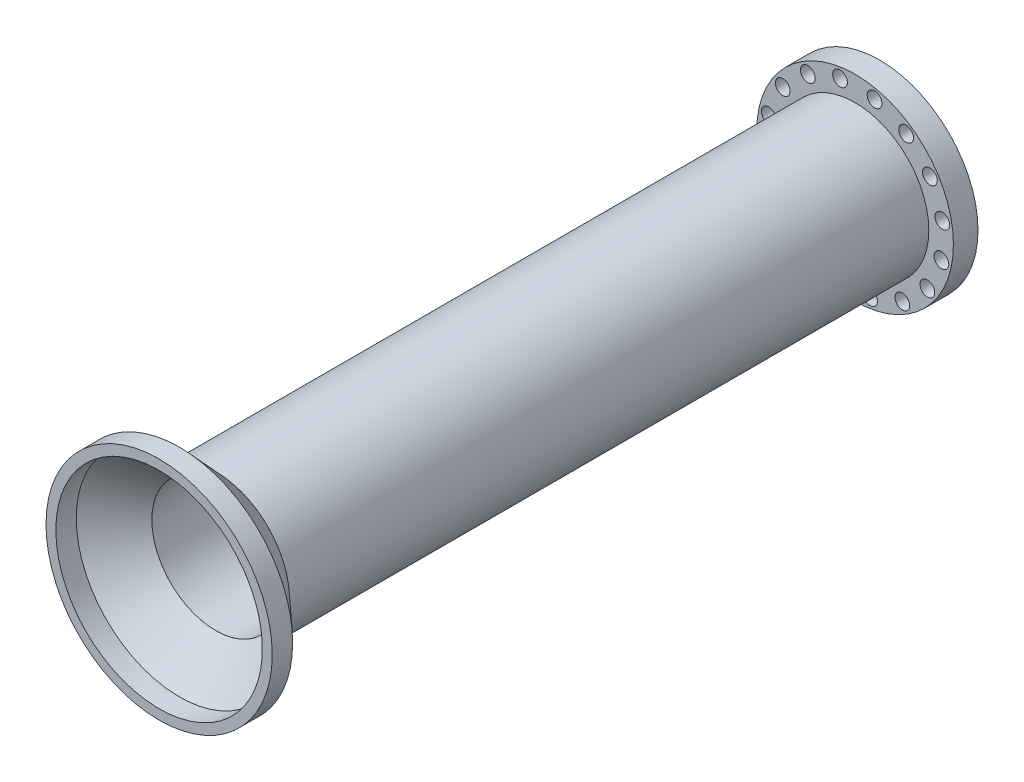
SolidWorks part; units mm, degrees
ref_plane "Front Plane" through (0, 0, 0) normal (0, 0, 1) x (1, 0, 0)
ref_plane "Top Plane" through (0, 0, 0) normal (0, 1, 0) x (1, 0, 0)
ref_plane "Right Plane" through (0, 0, 0) normal (1, 0, 0) x (0, 0, -1)
sketch "Sketch1" plane through (0, 0, 0) normal (0, 0, 1) x (1, 0, 0)
  line L1 (5, 78.5631) -> (35, 78.5631) construction
  circle A0 centre (20, 55.8305) radius 20
  circle A1 centre (20, 55.8305) radius 15
  point P5 (20, 78.5631)
  dimension "D1" = 40
  dimension "D2" = 30
extrude "Boss-Extrude1" add sketch "Sketch1" along normal blind 5 contours A1 | A0 A1
sketch "Sketch2" plane through (0, 0, 5) normal (0, 0, 1) x (1, 0, 0)
  circle A0 centre (20, 55.8305) radius 15
  circle A1 centre (20, 55.8305) radius 20 construction
  dimension "D1" = 5
extrude "Boss-Extrude2" add sketch "Sketch2" along normal blind 130
sketch "Sketch3" plane through (0, 0, 135) normal (0, 0, 1) x (1, 0, 0)
  circle A0 centre (20, 55.8305) radius 13
  circle A1 centre (20, 55.8305) radius 15 construction
  dimension "D1" = 2
extrude "Cut-Extrude1" cut sketch "Sketch3" against normal up to surface (130 mm away) and the other way through all up to face at (35, 55.8305, 5)
sketch "Sketch4" plane through (0, 0, 5) normal (0, 0, 1) x (1, 0, 0)
  circle A0 centre (20, 55.8305) radius 13
extrude "Cut-Extrude2" cut sketch "Sketch4" against normal through all
sketch "Sketch6" plane through (0, 0, 135) normal (0, 0, 1) x (1, 0, 0)
  line L0 (20, 70.8305) -> (20, 40.8305) construction
  circle A0 centre (20, 55.8305) radius 15 construction
ref_plane "Plane4" through (20, 0, 0) normal (-1, 0, 0) x (0, 0, 1)
sketch "Sketch7" plane through (20, 0, 0) normal (-1, 0, 0) x (0, 0, 1)
  line L1 (135, 55.8305) -> (146.019, 55.8305) construction
  line L5 (135, 68.8305) -> (135, 70.8305)
  line L6 (135, 70.8305) -> (135, 40.8305) construction
  line L10 (135, 42.8305) -> (135, 68.8305) construction
  line L11 (135, 70.8305) -> (142.3675, 78.8305)
  line L12 (142.3675, 78.8305) -> (146.5189, 78.8305)
  line L13 (146.5189, 78.8305) -> (146.5189, 76.8305)
  line L14 (146.5189, 76.8305) -> (142.3675, 76.8305)
  line L15 (142.3675, 76.8305) -> (135, 68.8305)
  dimension "D1" = 2
  dimension "D2" = 8
revolve "Revolve1" add sketch "Sketch7" angle 360 about L1
sketch "Sketch11" plane through (0, 0, 0) normal (0, 0, 1) x (1, 0, 0)
  circle A0 centre (20, 55.8305) radius 18 construction
  circle A2 centre (10.3884, 71.0495) radius 1.5
  circle A4 centre (16.9441, 73.5692) radius 1.5
  circle A5 centre (23.965, 73.3884) radius 1.5
  circle A6 centre (30.3823, 70.5345) radius 1.5
  circle A7 centre (35.219, 65.4421) radius 1.5
  circle A8 centre (37.7387, 58.8864) radius 1.5
  circle A9 centre (37.5579, 51.8655) radius 1.5
  circle A10 centre (34.704, 45.4482) radius 1.5
  circle A11 centre (29.6116, 40.6115) radius 1.5
  circle A12 centre (23.0559, 38.0918) radius 1.5
  circle A13 centre (16.035, 38.2726) radius 1.5
  circle A14 centre (9.6177, 41.1265) radius 1.5
  circle A15 centre (4.781, 46.2189) radius 1.5
  circle A16 centre (2.2613, 52.7746) radius 1.5
  circle A17 centre (2.4421, 59.7955) radius 1.5
  circle A18 centre (5.296, 66.2128) radius 1.5
  dimension "D1" = 36
  dimension "D2" = 3
  dimension "D3" = 16
extrude "Cut-Extrude4" cut sketch "Sketch11" along normal blind 50
